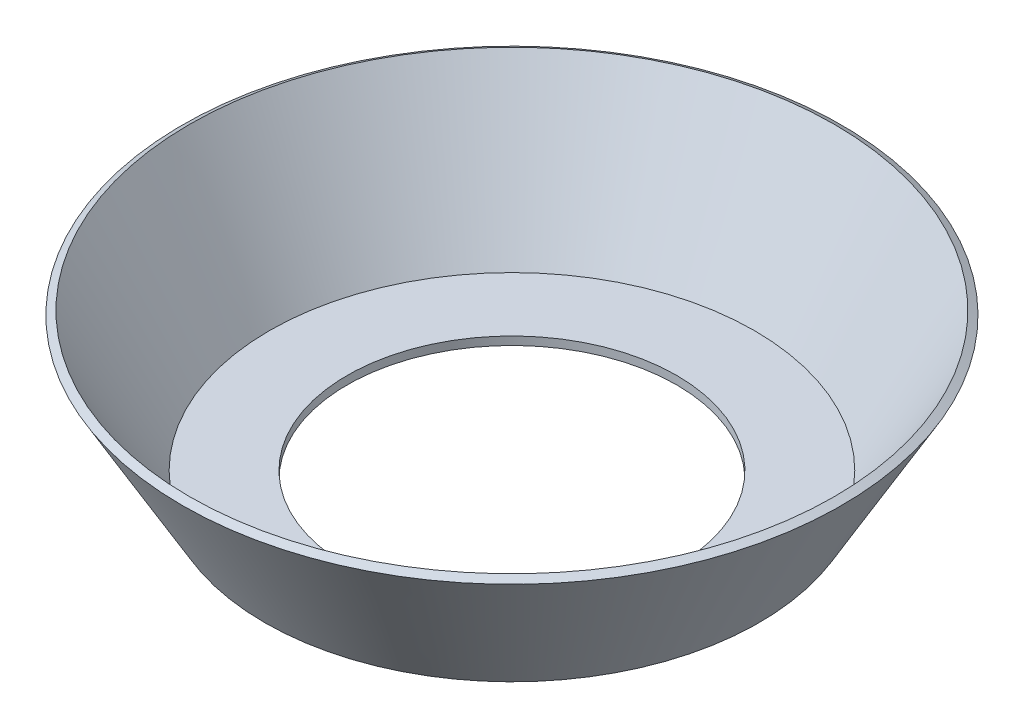
SolidWorks part; units mm, degrees
material "铝合金板 LF5"
ref_plane "Front Plane" through (0, 0, 0) normal (0, 0, 1) x (1, 0, 0)
ref_plane "Top Plane" through (0, 0, 0) normal (0, 1, 0) x (1, 0, 0)
ref_plane "Right Plane" through (0, 0, 0) normal (1, 0, 0) x (0, 0, -1)
sketch "Sketch1" plane through (0, 0, 0) normal (0, 0, 1) x (1, 0, 0)
  line L0 (0, 20.2632) -> (0, -31.8421) construction
  line L1 (10, 0) -> (15, 0)
  line L2 (15, 0) -> (20, 8.6603)
  line L3 (10, 0.5) -> (14.7113, 0.5)
  line L4 (14.7113, 0.5) -> (19.567, 8.9103)
  line L5 (10, 0.5) -> (10, 0)
  line L6 (19.567, 8.9103) -> (20, 8.6603)
  dimension "D1" = 20
  dimension "D2" = 5
  dimension "D3" = 120
  dimension "D5" = 10
  dimension "D4" = 0.5
revolve "Revolve1" add sketch "Sketch1" angle 360 about L0
